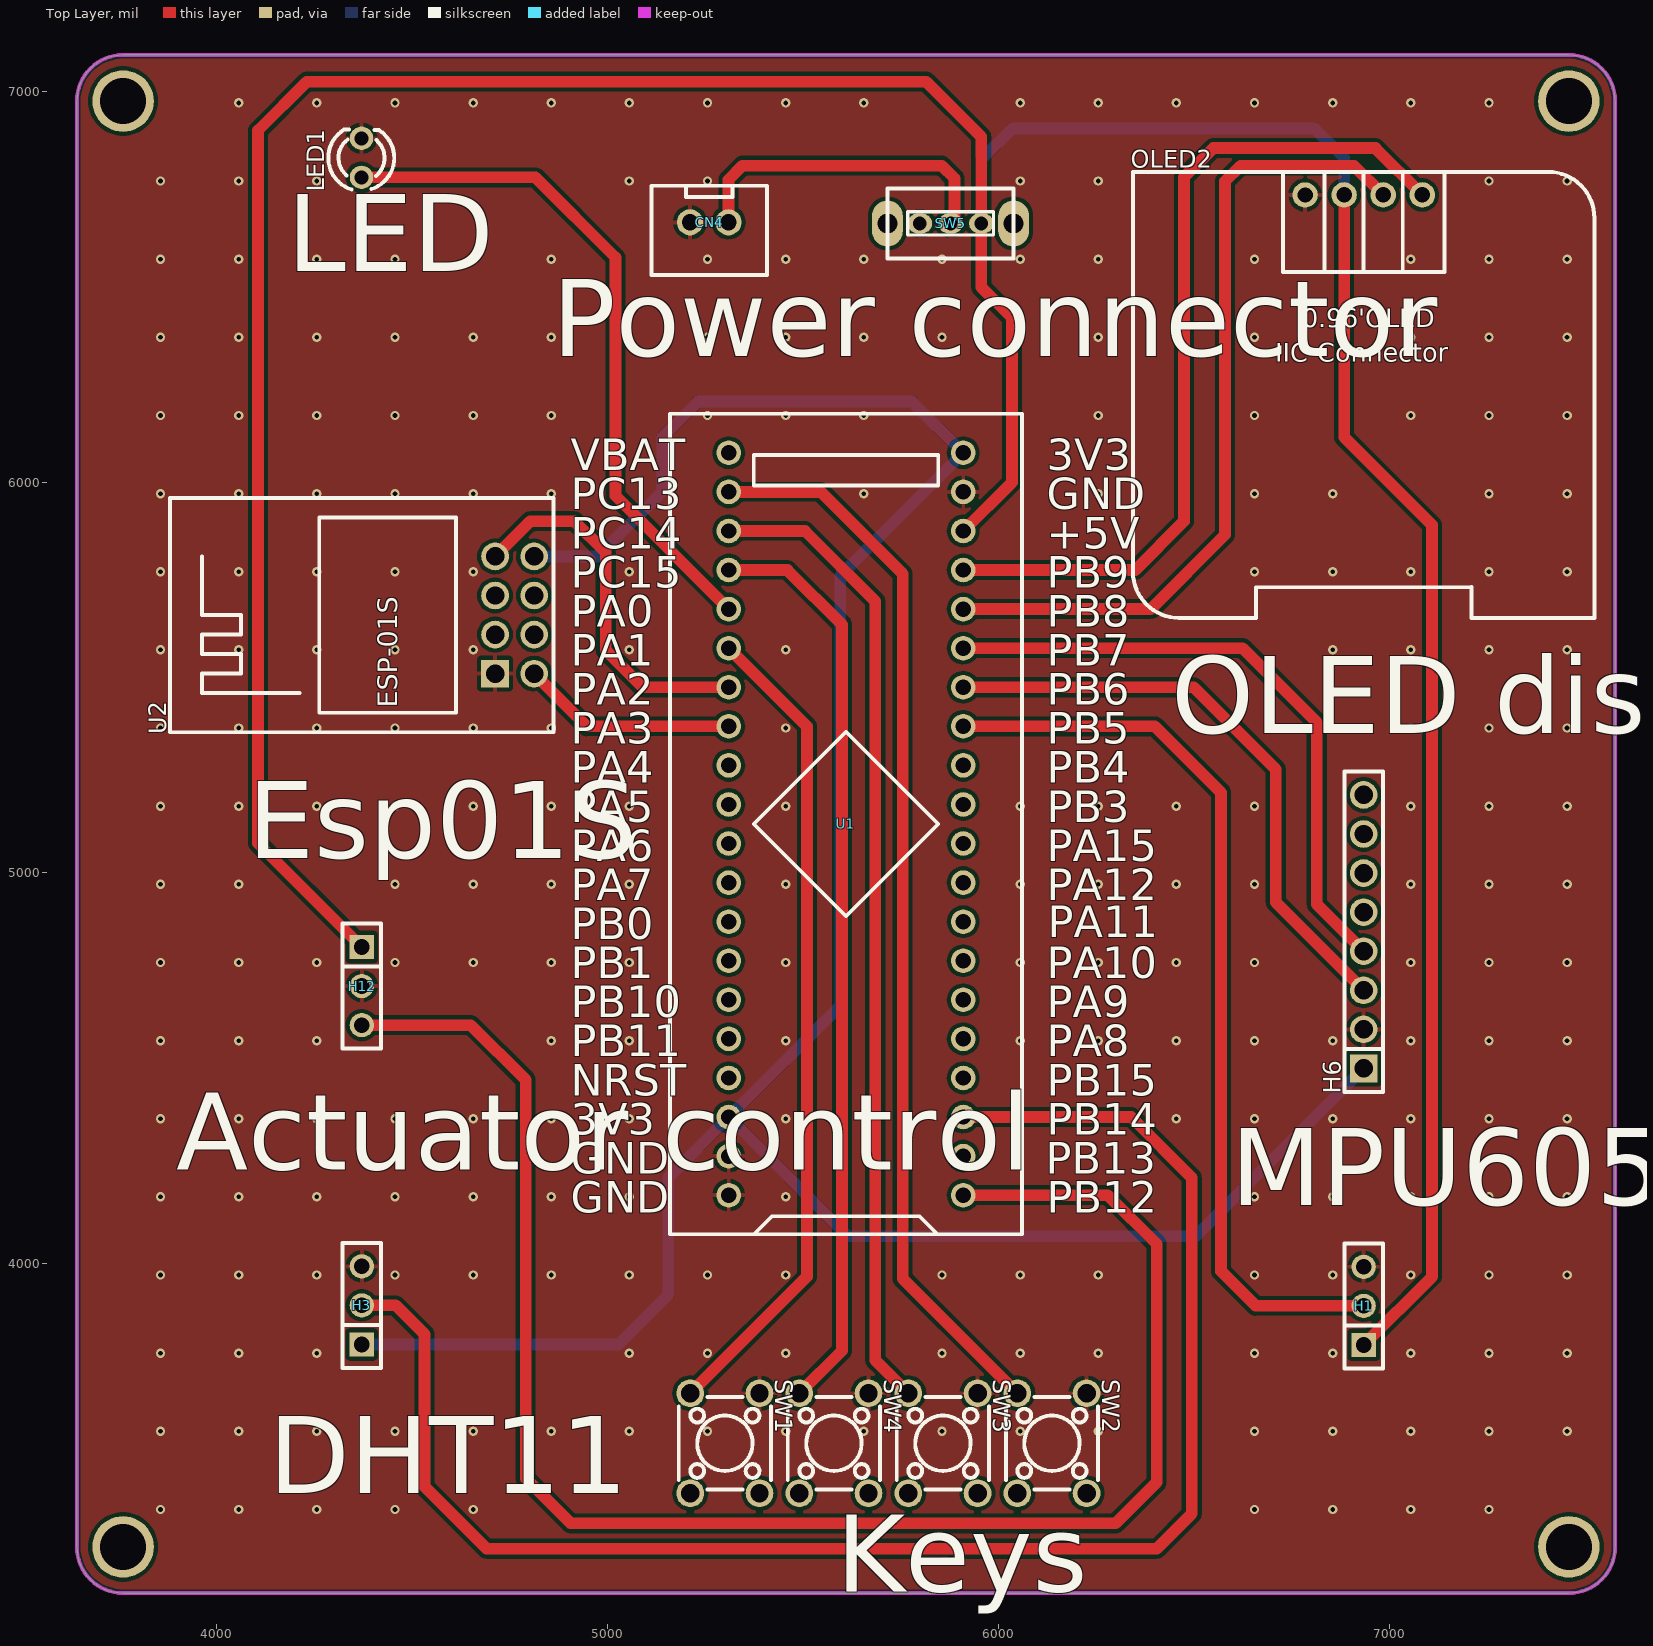
[diagram p0: Top Layer view]
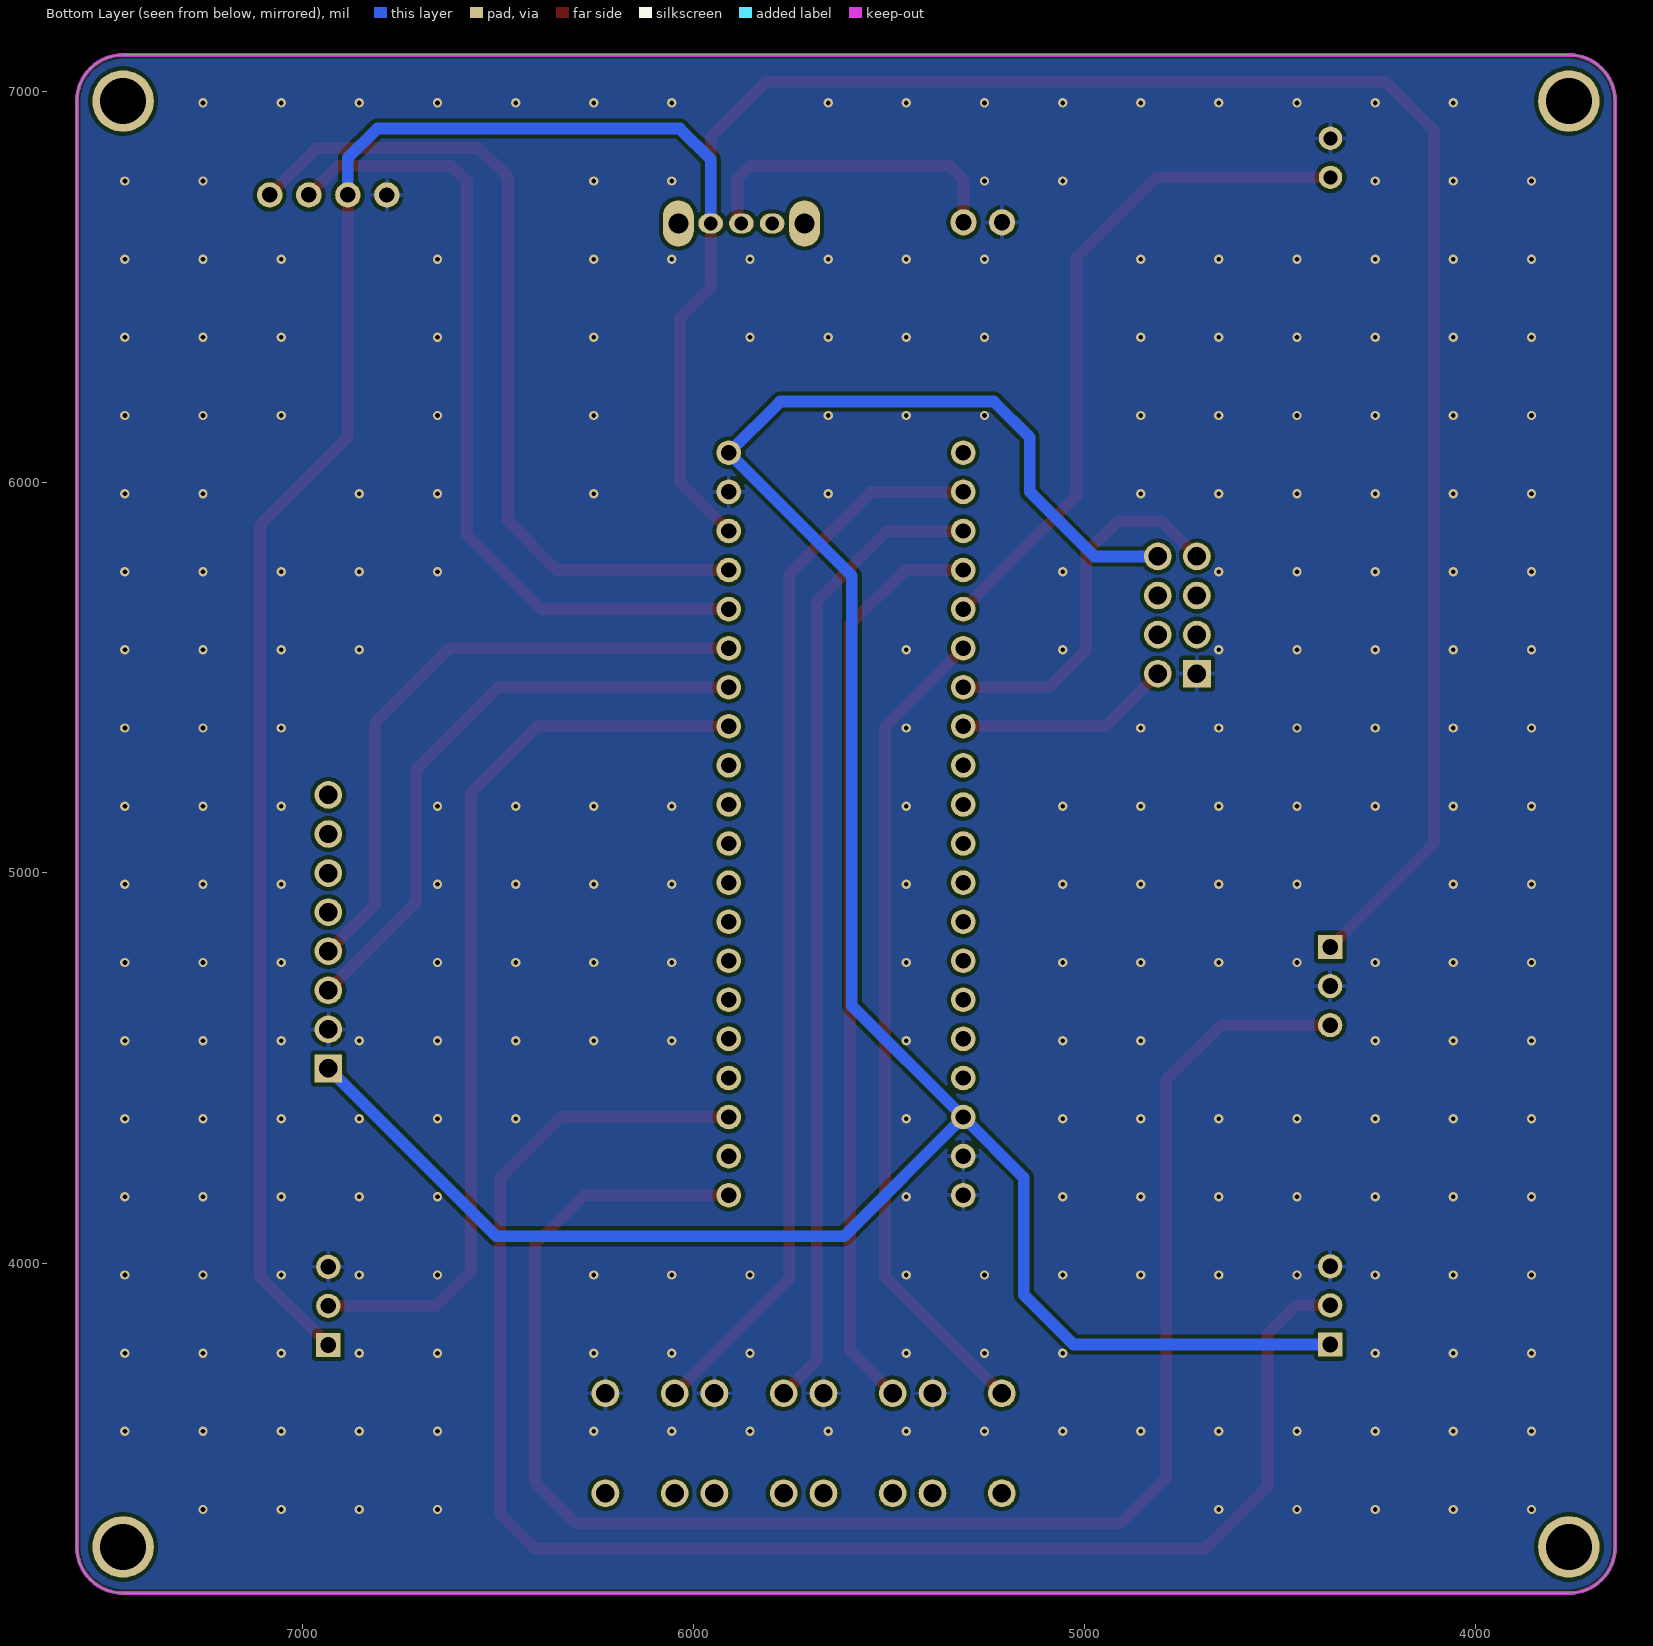
[diagram p1: Bottom Layer view, seen from below]
# Altium PCB MISC51555.pcbdoc
Units mil, origin at the board's own origin, x right, y up, seen from the top; angles counter-clockwise.
Board outline 3937.01 x 3937.01 mil, 2 copper layers (Top Layer, Bottom Layer), stack 62.206 mil thick; 14 components, 38 nets, 98 pads, 257 vias.

## Layer stack, top to bottom
Top Solder Mask Layer: solder mask 0.394, Dk 3.3
Top Layer: signal copper 1.379
Dielectric1: surface 59.449, FR4, Dk 4.5
Bottom Layer: signal copper 1.378
Bottom Solder Mask Layer: solder mask 0.394, Dk 3.3

## Board outline
3759.61,7093.5 ccw(c3759.61,6975.39) 3641.5,6975.39 3641.5,3274.61 ccw(c3759.61,3274.61) 3759.61,3156.5 7460.39,3156.5 ccw(c7460.39,3274.61) 7578.5,3274.61 7578.5,6975.39 ccw(c7460.39,6975.39) 7460.39,7093.5 3759.61,7093.5

## Design rules (kind name [scope] priority, off if disabled: settings)
BoardOutlineClearance copperThickness2oz_1 [All] p2 off: genericclearance=7.99 ignorepadtopadclearanceinfootprint=FALSE except(0: Arc-SplitContinuation Track-SplitContinuation SMDPad-SplitContinuation THPad-SplitContinuation Via-SplitContinuation Fill-SplitContinuation Region-SplitContinuation Poly-SplitContinuation Text-SplitContinuation Hole-SplitContinuation; 5.98: Arc-CutoutEdge Track-CutoutEdge SMDPad-CutoutEdge THPad-CutoutEdge Via-CutoutEdge Text-CutoutEdge; 6.9: Hole-OutlineEdge Hole-CutoutEdge; 10: Poly-OutlineEdge Poly-CutoutEdge; 11.81: Arc-OutlineEdge Track-OutlineEdge SMDPad-OutlineEdge THPad-OutlineEdge Via-OutlineEdge Fill-OutlineEdge Region-OutlineEdge Text-OutlineEdge Fill-CutoutEdge Region-CutoutEdge)
BoardOutlineClearance Plane_innerPlane_1 [All] p4 off: genericclearance=4.02 ignorepadtopadclearanceinfootprint=FALSE except(0: Arc-SplitContinuation Track-SplitContinuation SMDPad-SplitContinuation THPad-SplitContinuation Via-SplitContinuation Fill-SplitContinuation Region-SplitContinuation Poly-SplitContinuation Text-SplitContinuation Hole-SplitContinuation; 5.98: Arc-CutoutEdge Track-CutoutEdge SMDPad-CutoutEdge THPad-CutoutEdge Via-CutoutEdge Text-CutoutEdge; 6.9: Hole-OutlineEdge Hole-CutoutEdge; 10: Poly-OutlineEdge Poly-CutoutEdge; 11.81: Arc-OutlineEdge Track-OutlineEdge SMDPad-OutlineEdge THPad-OutlineEdge Via-OutlineEdge Fill-OutlineEdge Region-OutlineEdge Text-OutlineEdge Fill-CutoutEdge Region-CutoutEdge)
BoardOutlineClearance Copper_copperRegion_1 [All] p6 off: genericclearance=4.02 ignorepadtopadclearanceinfootprint=FALSE except(0: Arc-SplitContinuation Track-SplitContinuation SMDPad-SplitContinuation THPad-SplitContinuation Via-SplitContinuation Fill-SplitContinuation Region-SplitContinuation Poly-SplitContinuation Text-SplitContinuation Hole-SplitContinuation; 5.98: Arc-CutoutEdge Track-CutoutEdge SMDPad-CutoutEdge THPad-CutoutEdge Via-CutoutEdge Text-CutoutEdge; 6.9: Hole-OutlineEdge Hole-CutoutEdge; 10: Poly-OutlineEdge Poly-CutoutEdge; 11.81: Arc-OutlineEdge Track-OutlineEdge SMDPad-OutlineEdge THPad-OutlineEdge Via-OutlineEdge Fill-OutlineEdge Region-OutlineEdge Text-OutlineEdge Fill-CutoutEdge Region-CutoutEdge)
BoardOutlineClearance Copper_copperRegion_copperThickness1oz_1 [All] p8 off: genericclearance=4.02 ignorepadtopadclearanceinfootprint=FALSE except(0: Arc-SplitContinuation Track-SplitContinuation SMDPad-SplitContinuation THPad-SplitContinuation Via-SplitContinuation Fill-SplitContinuation Region-SplitContinuation Poly-SplitContinuation Text-SplitContinuation Hole-SplitContinuation; 5.98: Arc-CutoutEdge Track-CutoutEdge SMDPad-CutoutEdge THPad-CutoutEdge Via-CutoutEdge Text-CutoutEdge; 6.9: Hole-OutlineEdge Hole-CutoutEdge; 10: Poly-OutlineEdge Poly-CutoutEdge; 11.81: Arc-OutlineEdge Track-OutlineEdge SMDPad-OutlineEdge THPad-OutlineEdge Via-OutlineEdge Fill-OutlineEdge Region-OutlineEdge Text-OutlineEdge Fill-CutoutEdge Region-CutoutEdge)
BoardOutlineClearance Copper_copperRegion_Copper_copperRegion_1 [All] p10 off: genericclearance=4.02 ignorepadtopadclearanceinfootprint=FALSE except(0: Arc-SplitContinuation Track-SplitContinuation SMDPad-SplitContinuation THPad-SplitContinuation Via-SplitContinuation Fill-SplitContinuation Region-SplitContinuation Poly-SplitContinuation Text-SplitContinuation Hole-SplitContinuation; 5.98: Arc-CutoutEdge Track-CutoutEdge SMDPad-CutoutEdge THPad-CutoutEdge Via-CutoutEdge Text-CutoutEdge; 6.9: Hole-OutlineEdge Hole-CutoutEdge; 10: Poly-OutlineEdge Poly-CutoutEdge; 11.81: Arc-OutlineEdge Track-OutlineEdge SMDPad-OutlineEdge THPad-OutlineEdge Via-OutlineEdge Fill-OutlineEdge Region-OutlineEdge Text-OutlineEdge Fill-CutoutEdge Region-CutoutEdge)
BoardOutlineClearance copperThickness1oz_1 [All] p12: genericclearance=4.02 ignorepadtopadclearanceinfootprint=FALSE except(0: Arc-SplitContinuation Track-SplitContinuation SMDPad-SplitContinuation THPad-SplitContinuation Via-SplitContinuation Fill-SplitContinuation Region-SplitContinuation Poly-SplitContinuation Text-SplitContinuation Hole-SplitContinuation; 5.98: Arc-CutoutEdge Track-CutoutEdge SMDPad-CutoutEdge THPad-CutoutEdge Via-CutoutEdge Text-CutoutEdge; 6.9: Hole-OutlineEdge Hole-CutoutEdge; 10: Poly-OutlineEdge Poly-CutoutEdge; 11.81: Arc-OutlineEdge Track-OutlineEdge SMDPad-OutlineEdge THPad-OutlineEdge Via-OutlineEdge Fill-OutlineEdge Region-OutlineEdge Text-OutlineEdge Fill-CutoutEdge Region-CutoutEdge)
Clearance copperThickness2oz [All] p1 off: gap=7.99 ignorepadtopadclearanceinfootprint=FALSE except(5.98: SMDPad-Track SMDPad-SMDPad THPad-Track SMDPad-THPad THPad-THPad Track-Via SMDPad-Via THPad-Via Via-Via Fill-SMDPad Region-SMDPad Fill-THPad Region-THPad Fill-Via Region-Via Fill-Fill Fill-Region Region-Region Arc-Track Arc-SMDPad Arc-THPad Arc-Via Fill-Arc Region-Arc Arc-Arc Text-Track SMDPad-Text Text-THPad Text-Via Fill-Text Region-Text Arc-Text Text-Text; 6.9: Hole-Track Hole-SMDPad Hole-THPad Hole-Via Fill-Hole Region-Hole Hole-Arc Hole-Text; 10: Poly-Track Poly-SMDPad Poly-THPad Poly-Via Poly-Fill Poly-Region Poly-Poly Poly-Arc Poly-Text Poly-Hole; 11.81: Fill-Track Region-Track)
Clearance Plane_innerPlane [All] p3 off: gap=4.02 ignorepadtopadclearanceinfootprint=FALSE except(5.98: SMDPad-Track SMDPad-SMDPad THPad-Track SMDPad-THPad THPad-THPad Track-Via SMDPad-Via THPad-Via Via-Via Fill-SMDPad Region-SMDPad Fill-THPad Region-THPad Fill-Via Region-Via Fill-Fill Fill-Region Region-Region Arc-Track Arc-SMDPad Arc-THPad Arc-Via Fill-Arc Region-Arc Arc-Arc Text-Track SMDPad-Text Text-THPad Text-Via Fill-Text Region-Text Arc-Text Text-Text; 6.9: Hole-Track Hole-SMDPad Hole-THPad Hole-Via Fill-Hole Region-Hole Hole-Arc Hole-Text; 10: Poly-Track Poly-SMDPad Poly-THPad Poly-Via Poly-Fill Poly-Region Poly-Poly Poly-Arc Poly-Text Poly-Hole; 11.81: Fill-Track Region-Track)
Clearance Copper_copperRegion [All] p5 off: gap=4.02 ignorepadtopadclearanceinfootprint=FALSE except(5.98: SMDPad-Track SMDPad-SMDPad THPad-Track SMDPad-THPad THPad-THPad Track-Via SMDPad-Via THPad-Via Via-Via Fill-SMDPad Region-SMDPad Fill-THPad Region-THPad Fill-Via Region-Via Fill-Fill Fill-Region Region-Region Arc-Track Arc-SMDPad Arc-THPad Arc-Via Fill-Arc Region-Arc Arc-Arc Text-Track SMDPad-Text Text-THPad Text-Via Fill-Text Region-Text Arc-Text Text-Text; 6.9: Hole-Track Hole-SMDPad Hole-THPad Hole-Via Fill-Hole Region-Hole Hole-Arc Hole-Text; 10: Poly-Track Poly-SMDPad Poly-THPad Poly-Via Poly-Fill Poly-Region Poly-Poly Poly-Arc Poly-Text Poly-Hole; 11.81: Fill-Track Region-Track)
Clearance Copper_copperRegion_copperThickness1oz [All] p7 off: gap=4.02 ignorepadtopadclearanceinfootprint=FALSE except(5.98: SMDPad-Track SMDPad-SMDPad THPad-Track SMDPad-THPad THPad-THPad Track-Via SMDPad-Via THPad-Via Via-Via Fill-SMDPad Region-SMDPad Fill-THPad Region-THPad Fill-Via Region-Via Fill-Fill Fill-Region Region-Region Arc-Track Arc-SMDPad Arc-THPad Arc-Via Fill-Arc Region-Arc Arc-Arc Text-Track SMDPad-Text Text-THPad Text-Via Fill-Text Region-Text Arc-Text Text-Text; 6.9: Hole-Track Hole-SMDPad Hole-THPad Hole-Via Fill-Hole Region-Hole Hole-Arc Hole-Text; 10: Poly-Track Poly-SMDPad Poly-THPad Poly-Via Poly-Fill Poly-Region Poly-Poly Poly-Arc Poly-Text Poly-Hole; 11.81: Fill-Track Region-Track)
Clearance Copper_copperRegion_Copper_copperRegion [All] p9 off: gap=4.02 ignorepadtopadclearanceinfootprint=FALSE except(5.98: SMDPad-Track SMDPad-SMDPad THPad-Track SMDPad-THPad THPad-THPad Track-Via SMDPad-Via THPad-Via Via-Via Fill-SMDPad Region-SMDPad Fill-THPad Region-THPad Fill-Via Region-Via Fill-Fill Fill-Region Region-Region Arc-Track Arc-SMDPad Arc-THPad Arc-Via Fill-Arc Region-Arc Arc-Arc Text-Track SMDPad-Text Text-THPad Text-Via Fill-Text Region-Text Arc-Text Text-Text; 6.9: Hole-Track Hole-SMDPad Hole-THPad Hole-Via Fill-Hole Region-Hole Hole-Arc Hole-Text; 10: Poly-Track Poly-SMDPad Poly-THPad Poly-Via Poly-Fill Poly-Region Poly-Poly Poly-Arc Poly-Text Poly-Hole; 11.81: Fill-Track Region-Track)
Clearance copperThickness1oz [All] p11: gap=4.02 ignorepadtopadclearanceinfootprint=FALSE except(5.98: SMDPad-Track SMDPad-SMDPad THPad-Track SMDPad-THPad THPad-THPad Track-Via SMDPad-Via THPad-Via Via-Via Fill-SMDPad Region-SMDPad Fill-THPad Region-THPad Fill-Via Region-Via Fill-Fill Fill-Region Region-Region Arc-Track Arc-SMDPad Arc-THPad Arc-Via Fill-Arc Region-Arc Arc-Arc Text-Track SMDPad-Text Text-THPad Text-Via Fill-Text Region-Text Arc-Text Text-Text; 6.9: Hole-Track Hole-SMDPad Hole-THPad Hole-Via Fill-Hole Region-Hole Hole-Arc Hole-Text; 10: Poly-Track Poly-SMDPad Poly-THPad Poly-Via Poly-Fill Poly-Region Poly-Poly Poly-Arc Poly-Text Poly-Hole; 11.81: Fill-Track Region-Track)
DiffPairsRouting differentialPair [All] p1: maxlimit=6 minlimit=6 mostfreqgap=6 toplayer_minwidth=5 toplayer_prefwidth=10 toplayer_maxwidth=100 toplayer_mingap=6 toplayer_prefgap=6 toplayer_maxgap=6 bottomlayer_minwidth=5 bottomlayer_prefwidth=10 bottomlayer_maxwidth=100 bottomlayer_mingap=6 bottomlayer_prefgap=6 bottomlayer_maxgap=6 maxuncoupledlength=10
HoleToHoleClearance otherClearance [All] p1: gap=11.81 allowstackedmicrovias=TRUE
Length netLength [All] p1: minlimit=0 maxlimit=0
PasteMaskExpansion pasteMaskExpansion [All] p1: expansion=0
PlaneConnect innerPlane [All] p1: planeconnectstyle=Relief reliefexpansion=20 reliefentries=4 reliefconductorwidth=10 reliefairgap=10
PolygonConnect copperRegion_copperThickness1oz [All] p1 off: connectstyle=Relief reliefconductorwidth=10 reliefentries=4 polygonreliefangle="90 Angle" airgapwidth=10 via.connectstyle=Relief via.reliefconductorwidth=10 via.reliefentries=4 via.polygonreliefangle="90 Angle" via.airgapwidth=10
PolygonConnect copperRegion_Copper_copperRegion [All] p2 off: connectstyle=Relief reliefconductorwidth=10 reliefentries=4 polygonreliefangle="90 Angle" airgapwidth=10 via.connectstyle=Relief via.reliefconductorwidth=10 via.reliefentries=4 via.polygonreliefangle="90 Angle" via.airgapwidth=10
PolygonConnect copperRegion [All] p3: connectstyle=Relief reliefconductorwidth=10 reliefentries=4 polygonreliefangle="90 Angle" airgapwidth=10 via.connectstyle=Relief via.reliefconductorwidth=10 via.reliefentries=4 via.polygonreliefangle="90 Angle" via.airgapwidth=10
RoutingVias viaSize [All] p1: holewidth=12.01 width=24.02 viastyle="Through Hole" minholewidth=11.81 minwidth=19.68 maxholewidth=248.03 maxwidth=393.7
SolderMaskExpansion solderMaskExpansion [IsVia] p1: expansion=-1000 istentingtop=TRUE
SolderMaskExpansion solderMaskExpansion [All] p2: expansion=2 istentingtop=FALSE
Width copperThickness2oz_2 [All] p1 off: maxlimit=100 minlimit=8 preferedwidth=10
Width copperThickness1oz_2 [All] p2: maxlimit=100 minlimit=5 preferedwidth=10

## Components (designator, comment, footprint, x,y, rotation, side; value= is the part's Value field where it differs from the comment)
CN4 "XH2.54*2P_THT" CONN-TH_2P-P2.50-XH2.54-2P 5260,6665 r0 top
H1 "" HDR-TH_3P-P2.54-V-F 6935,3891.7 r90 top
H3 "" HDR-TH_3P-P2.54-V-F 4370.79,3892.91 r90 top
H6 "" HDR-TH_8P-P2.54-V-F-1 6934.99,4849.41 r90 top
H12 "" HDR-TH_3P-P2.54-V-F 4370.79,4710.2 r270 top
LED1 "" LED_TH-3mm 4370,6830 r90 top
OLED2 "" 0.96OLED_4P 6935,6735 r0 top
SW1 "" SW-TH_4P-L6.0-W6.0-P4.50-LS6.5 5300,3540 r270 top
SW2 "" SW-TH_4P-L6.0-W6.0-P4.50-LS6.5 6137.14,3540 r270 top
SW3 "" SW-TH_4P-L6.0-W6.0-P4.50-LS6.5 5858.09,3540 r270 top
SW4 "" SW-TH_4P-L6.0-W6.0-P4.50-LS6.5 5579.05,3540 r270 top
SW5 "" 拨动开关 5882.9,6662.05 r180 top
U1 "STM32F103C8T6-Card" CONN-TH_L53.3-W22.9_STM32F103C8T6-CARD 5610,5125 r90 top
U2 "ESP-01S" WIFIM-TH_ESP-01S 4761.79,5659.81 r90 top

## Footprints (in the part's own frame and the unit in brackets; to place one, negate y for a bottom-side part, rotate by r counter-clockwise, add the part's x,y. Pads: shape width x height; smd on the part's side, far side on the other; paste and mask are expansions set on the pad)
0.96OLED_4P [mm]
  round 1.65 hole 1 copper offset 0,0: 1(-3.81,-0.001) 2(-1.27,0.002) 3(1.27,0.002) 4(3.81,0.002)
  silkscreen extent -15,-27.5 15,1.5
CONN-TH_2P-P2.50-XH2.54-2P [mm]
  round 1.7 hole 1.05 paste+0 mask+0.05: 1(1.25,0) 2(-1.25,0)
  silkscreen extent -3.75,-3.42 3.75,2.37
CONN-TH_L53.3-W22.9_STM32F103C8T6-CARD [mm]
  round 1.6 hole 1: 1(-24.13,-7.62) 2(-21.59,-7.62) 3(-19.05,-7.62) 4(-16.51,-7.62) 5(-13.97,-7.62) 6(-11.43,-7.62) 7(-8.89,-7.62) 8(-6.35,-7.62) 9(-3.81,-7.62) 10(-1.27,-7.62) 11(1.27,-7.62) 12(3.81,-7.62) 13(6.35,-7.62) 14(8.89,-7.62) 15(11.43,-7.62) 16(13.97,-7.62) 17(16.51,-7.62) 18(19.05,-7.62) 19(21.59,-7.62) 20(24.13,-7.62) 21(24.13,7.62) 22(21.59,7.62) 23(19.05,7.62) 24(16.51,7.62) 25(13.97,7.62) 26(11.43,7.62) 27(8.89,7.62) 28(6.35,7.62) 29(3.81,7.62) 30(1.27,7.62) 31(-1.27,7.62) 32(-3.81,7.62) 33(-6.35,7.62) 34(-8.89,7.62) 35(-11.43,7.62) 36(-13.97,7.62) 37(-16.51,7.62) 38(-19.05,7.62) 39(-21.59,7.62) 40(-24.13,7.62)
  silkscreen extent -26.67,-11.43 26.67,11.43
HDR-TH_3P-P2.54-V-F [mil]
  rect 62x62 hole 40.16: 1(-100,0)
  round 62 hole 40.16: 2(0,0) 3(100,0)
  silkscreen extent -160,-49 160,49
HDR-TH_8P-P2.54-V-F-1 [mm]
  rect 1.8x1.8 hole 1.2: 1(-8.89,0)
  round 1.8 hole 1.2: 2(-6.35,0) 3(-3.81,0) 4(-1.27,0) 5(1.27,0) 6(3.81,0) 7(6.35,0) 8(8.89,0)
  silkscreen extent -10.41,-1.25 10.41,1.25
LED_TH-3mm [mil]
  round 60 hole 36 paste+0 mask+2: 1(-50,0) 2(50,0)
  silkscreen extent -81,-84 72,85
SW-TH_4P-L6.0-W6.0-P4.50-LS6.5 [mm]
  round 1.8 hole 1.2: 1(-3.25,2.25) 2(3.25,2.25) 3(-3.25,-2.25) 4(3.25,-2.25)
  silkscreen extent -3,-3 3,3
WIFIM-TH_ESP-01S [mm]
  rect 1.8x1.8 hole 1.2: 1(-3.81,1.27)
  round 1.8 hole 1.2: 2(-1.27,1.27) 3(1.27,1.27) 4(3.81,1.27) 5(3.81,-1.27) 6(1.27,-1.27) 7(-1.27,-1.27) 8(-3.81,-1.27)
  silkscreen extent -7.62,-2.54 7.62,22.4
拨动开关 [mil]
  oval 63x51.2 hole 35.4 paste+0 mask+2: 1(-73.4,0) 2(5,0) 3(84,0)
  oval 78.7x118.1 hole 51.2 paste+0 mask+2: 4(166.7,0) 5(-156.1,0)
  silkscreen extent -156,-90 167,90

## Free pads (board coordinates)
  round 157.48 hole 118.11: 1(3759.61,6975.39) 1(3759.61,3274.61) 1(7460.39,6975.39) 1(7460.39,3274.61)

## Via types
v1: diameter 24.02, hole 12, Top Layer to Bottom Layer, 257 vias

## Nets (pads, with @x,y where several pads share a name; then routed paths per layer and width w, separated by ;. In a path a pad name is that pad's centre, name@x,y a point inside that pad or via, vN(x,y) a via of type N, cw(c..) or ccw(c..) an arc to the next point about the centre after c; other vN are vias at no path point)
$1N17118: CN4.1 SW5.2 | length 831.4
  Top Layer w30: CN4.1 5309.22,6774.22 5345,6810 5855,6810 5887.9,6777.1 SW5.2@5887.9,6662.05
+5V: H1.1 H12.1 OLED2.2 SW5.1 U1.18 | length 9615.2
  Top Layer w30: H12.1 4105,5075.99 4105,6900 4230,7025 5815,7025 5956.3,6883.7 SW5.1 5956.3,6498.7 6035,6420 6035,6000 U1.18 ; OLED2.2@6885,6735.05 6885,6115 7110,5890 7110,3966.7 H1.1
  Bottom Layer w30: SW5.1 5956.3,6826.3 6035,6905 6810,6905 6885,6830 OLED2.2@6885,6735.05
GND: CN4.2 H1.3 H3.3 H6.2 H12.2 LED1.2 OLED2.1 SW1.1 SW2.1 SW3.1 SW4.1 U1.19 U1.39 U1.40 U2.1
  other v1: 3855.6,3370.6 4055.6,3370.6 4255.6,3370.6 4455.6,3370.6 4655.6,3370.6 6655.6,3370.6 6855.6,3370.6 7055.6,3370.6 7255.6,3370.6 3855.6,3570.6 4055.6,3570.6 4255.6,3570.6 4455.6,3570.6 4655.6,3570.6 4855.6,3570.6 5055.6,3570.6 5255.6,3570.6 5455.6,3570.6 5655.6,3570.6 5855.6,3570.6 6055.6,3570.6 6255.6,3570.6 6655.6,3570.6 6855.6,3570.6 7055.6,3570.6 7255.6,3570.6 7455.6,3570.6 3855.6,3770.6 4055.6,3770.6 4255.6,3770.6 5055.6,3770.6 5255.6,3770.6 5455.6,3770.6 5855.6,3770.6 6055.6,3770.6 6255.6,3770.6 6655.6,3770.6 6855.6,3770.6 7055.6,3770.6 7255.6,3770.6 7455.6,3770.6 3855.6,3970.6 4055.6,3970.6 4255.6,3970.6 4455.6,3970.6 4655.6,3970.6 4855.6,3970.6 5055.6,3970.6 5255.6,3970.6 5455.6,3970.6 5855.6,3970.6 6055.6,3970.6 6255.6,3970.6 6655.6,3970.6 6855.6,3970.6 7055.6,3970.6 7255.6,3970.6 7455.6,3970.6 3855.6,4170.6 4055.6,4170.6 4255.6,4170.6 4455.6,4170.6 4655.6,4170.6 4855.6,4170.6 5055.6,4170.6 5455.6,4170.6 6655.6,4170.6 6855.6,4170.6 7055.6,4170.6 7255.6,4170.6 7455.6,4170.6 3855.6,4370.6 4055.6,4370.6 4255.6,4370.6 4455.6,4370.6 4655.6,4370.6 4855.6,4370.6 5055.6,4370.6 5455.6,4370.6 6455.6,4370.6 6655.6,4370.6 6855.6,4370.6 7055.6,4370.6 7255.6,4370.6 7455.6,4370.6 3855.6,4570.6 4055.6,4570.6 4255.6,4570.6 4855.6,4570.6 5055.6,4570.6 5455.6,4570.6 6055.6,4570.6 6255.6,4570.6 6455.6,4570.6 6655.6,4570.6 6855.6,4570.6 7055.6,4570.6 7255.6,4570.6 7455.6,4570.6 3855.6,4770.6 4055.6,4770.6 4255.6,4770.6 4455.6,4770.6 4655.6,4770.6 4855.6,4770.6 5055.6,4770.6 5455.6,4770.6 6055.6,4770.6 6255.6,4770.6 6455.6,4770.6 6655.6,4770.6 7055.6,4770.6 7255.6,4770.6 7455.6,4770.6 3855.6,4970.6 4055.6,4970.6 4455.6,4970.6 4655.6,4970.6 4855.6,4970.6 5055.6,4970.6 5455.6,4970.6 6055.6,4970.6 6255.6,4970.6 6455.6,4970.6 6655.6,4970.6 7055.6,4970.6 7255.6,4970.6 7455.6,4970.6 3855.6,5170.6 4055.6,5170.6 4255.6,5170.6 4455.6,5170.6 4655.6,5170.6 4855.6,5170.6 5055.6,5170.6 5455.6,5170.6 6055.6,5170.6 6255.6,5170.6 6455.6,5170.6 6655.6,5170.6 7055.6,5170.6 7255.6,5170.6 7455.6,5170.6 3855.6,5370.6 4055.6,5370.6 4255.6,5370.6 4455.6,5370.6 4655.6,5370.6 4855.6,5370.6 5455.6,5370.6 7055.6,5370.6 7255.6,5370.6 7455.6,5370.6 3855.6,5570.6 4055.6,5570.6 4255.6,5570.6 4455.6,5570.6 4655.6,5570.6 5055.6,5570.6 5455.6,5570.6 6855.6,5570.6 7055.6,5570.6 7255.6,5570.6 7455.6,5570.6 3855.6,5770.6 4055.6,5770.6 4255.6,5770.6 4455.6,5770.6 4655.6,5770.6 5055.6,5770.6 6655.6,5770.6 6855.6,5770.6 7055.6,5770.6 7255.6,5770.6 7455.6,5770.6 3855.6,5970.6 4055.6,5970.6 4255.6,5970.6 4455.6,5970.6 4655.6,5970.6 4855.6,5970.6 5655.6,5970.6 6255.6,5970.6 6655.6,5970.6 6855.6,5970.6 7255.6,5970.6 7455.6,5970.6 3855.6,6170.6 4055.6,6170.6 4255.6,6170.6 4455.6,6170.6 4655.6,6170.6 4855.6,6170.6 5255.6,6170.6 5455.6,6170.6 5655.6,6170.6 6255.6,6170.6 6655.6,6170.6 7055.6,6170.6 7255.6,6170.6 7455.6,6170.6 3855.6,6370.6 4055.6,6370.6 4255.6,6370.6 4455.6,6370.6 4655.6,6370.6 4855.6,6370.6 5255.6,6370.6 5455.6,6370.6 5655.6,6370.6 5855.6,6370.6 6255.6,6370.6 6655.6,6370.6 7055.6,6370.6 7255.6,6370.6 7455.6,6370.6 3855.6,6570.6 4055.6,6570.6 4255.6,6570.6 4455.6,6570.6 4655.6,6570.6 4855.6,6570.6 5255.6,6570.6 5455.6,6570.6 5655.6,6570.6 5855.6,6570.6 6055.6,6570.6 6255.6,6570.6 6655.6,6570.6 7055.6,6570.6 7255.6,6570.6 7455.6,6570.6 3855.6,6770.6 4055.6,6770.6 4255.6,6770.6 5055.6,6770.6 5255.6,6770.6 6055.6,6770.6 6255.6,6770.6 7255.6,6770.6 7455.6,6770.6 4055.6,6970.6 4255.6,6970.6 4455.6,6970.6 4655.6,6970.6 4855.6,6970.6 5055.6,6970.6 5255.6,6970.6 5455.6,6970.6 5655.6,6970.6 6055.6,6970.6 6255.6,6970.6 6455.6,6970.6 6655.6,6970.6 6855.6,6970.6 7055.6,6970.6 7255.6,6970.6
NRST: U1.37
PA0: LED1.1 U1.25 | length 1755
  Top Layer w30: LED1.1 4815,6780 5020,6575 5020,5965 U1.25
PA1: SW1.3 U1.26 | length 2113.6
  Top Layer w30: SW1.3 5510,3966.53 5510,5375 U1.26
PA2: U1.27 U2.4 | length 958.1
  Top Layer w30: U2.4 4801.97,5900 4915,5900 4995,5820 4995,5570 5090,5475 U1.27
PA3: U1.28 U2.8 | length 554.1
  Top Layer w30: U2.8 4946.6,5375 U1.28
PA4: U1.29
PA5: U1.30
PA6: U1.31
PA7: U1.32
PA8: U1.5
PA9: U1.6
PA10: U1.7
PA11: U1.8
PA12: U1.9
PA15: U1.10
PB0: U1.33
PB1: U1.34
PB3: U1.11
PB4: U1.12
PB5: H1.2 U1.13 | length 2357
  Top Layer w30: U1.13 6400,5375 6570,5205 6570,3980 6658.31,3891.7 H1.2
PB6: H6.3 U1.14 | length 1545.8
  Top Layer w30: U1.14 6500,5475 6710,5265 6710,4924.41 H6.3
PB7: H6.4 U1.15 | length 1619
  Top Layer w30: U1.15 6625,5575 6815,5385 6815,4919.41 H6.4
PB8: OLED2.3 U1.16 | length 2106.3
  Top Layer w30: U1.16 6390,5675 6580,5865 6580,6770 6620,6810 6910.05,6810 OLED2.3@6985,6735.05
PB9: OLED2.4 U1.17 | length 2187.5
  Top Layer w30: U1.17 6350,5775 6475,5900 6475,6780 6550,6855 6965.05,6855 OLED2.4@7085,6735.05
PB10: U1.35
PB11: U1.36
PB12: H12.3 U1.1 | length 4360.2
  Top Layer w30: H12.3 4649.8,4610.2 4790,4470 4790,3450 4905,3335 6300,3335 6405,3440 6405,4050 6280,4175 U1.1
PB13: U1.2
PB14: H3.2 U1.3 | length 4157.2
  Top Layer w30: H3.2 4457.09,3892.91 4531.44,3818.56 4531.44,3428.56 4690,3270 6405,3270 6495,3360 6495,4220 6340,4375 U1.3
PB15: U1.4
PC13: SW2.3 U1.22 | length 2750.6
  Top Layer w30: U1.22 5545,5975 5755,5765 5755,3961.51 SW2.3
PC14: SW3.3 U1.23 | length 2511.6
  Top Layer w30: U1.23 5505,5875 5685,5695 5685,3752.46 SW3.3
PC15: SW4.3 U1.24 | length 2360.4
  Top Layer w30: U1.24 5460,5775 5600,5635 5600,3777.48 SW4.3
VBAT: U1.21
VCC: H3.1 H6.1 U1.20 U1.38 U2.5 | length 6632.6
  Bottom Layer w30: H3.1 5027.91,3792.91 5155,3920 5155,4220 U1.38 ; U2.5 4974.81,5809.81 5140,5975 5140,6115 5231.21,6206.21 5778.79,6206.21 U1.20 5595,5760 5595,4660 U1.38 ; H6.1 6505.58,4070 5615,4070 U1.38
pads on no net: H6.5 H6.6 H6.7 H6.8 SW1.2 SW1.4 SW2.2 SW2.4 SW3.2 SW3.4 SW4.2 SW4.4 SW5.3 SW5.4 SW5.5 U2.2 U2.3 U2.6 U2.7

## Polygon pours and split planes (outlines as drawn)
GND on Bottom Layer (solid, remove dead copper, pour order 2): 3570,7215 3570,3050 7745,3050 7745,7215
GND on Top Layer (solid, remove dead copper, pour order 2): 3000,7415 3000,3000 7930,3000 7930,7415

## Keep-outs
Board Outline Layer:
  the board outline again, w10

## Silkscreen, mask and mechanical layers (free items; w line width, h text height)
Top Silkscreen Layer:
  text "LED" at 4180,6540 h196.85
  text "Power connector" at 4857.87,6321.57 h196.85
  text "VBAT" at 4905.95,6030 h80
  text "3V3" at 6124.16,6030 h80
  text "PC13" at 4905.95,5930 h80
  text "GND" at 6124.16,5930 h80
  text "PC14" at 4905.95,5830 h80
  text "+5V" at 6124.16,5830 h80
  text "PC15" at 4905.95,5730 h80
  text "PB9" at 6124.16,5730 h80
  text "PA0" at 4905.95,5630 h80
  text "PB8" at 6124.16,5630 h80
  text "PA1" at 4905.95,5530 h80
  text "PB7" at 6124.16,5530 h80
  text "PA2" at 4905.95,5430 h80
  text "PB6" at 6124.16,5430 h80
  text "OLED display" at 6443.02,5357.38 h196.85
  text "PA3" at 4905.95,5330 h80
  text "PB5" at 6124.16,5330 h80
  text "PA4" at 4905.95,5230 h80
  text "PB4" at 6124.16,5230 h80
  text "PA5" at 4905.95,5130 h80
  text "PB3" at 6124.16,5130 h80
  text "Esp01S" at 4078.49,5037.42 h196.85
  text "PA6" at 4905.95,5030 h80
  text "PA15" at 6124.16,5030 h80
  text "PA7" at 4905.95,4930 h80
  text "PA12" at 6124.16,4930 h80
  text "PA11" at 6125.95,4835 h80
  text "PB0" at 4905.95,4830 h80
  text "PB1" at 4905.95,4730 h80
  text "PA10" at 6124.16,4730 h80
  text "PB10" at 4905.95,4630 h80
  text "PA9" at 6124.16,4630 h80
  text "PB11" at 4905.95,4530 h80
  text "PA8" at 6124.16,4530 h80
  text "NRST" at 4905.95,4430 h80
  text "PB15" at 6124.16,4430 h80
  text "3V3" at 4905.95,4330 h80
  text "PB14" at 6124.16,4330 h80
  text "Actuator control" at 3895.77,4240 h196.85
  text "GND" at 4905.95,4230 h80
  text "PB13" at 6120.95,4230 h80
  text "MPU6050" at 6594.68,4149.07 h196.85
  text "GND" at 4905.95,4130 h80
  text "PB12" at 6124.16,4130 h80
  text "Sound and light alarm module" at 6342.95,3450 h196.85
  text "DHT11" at 4132.18,3411.68 h196.85
  text "Keys" at 5585,3160 h196.85